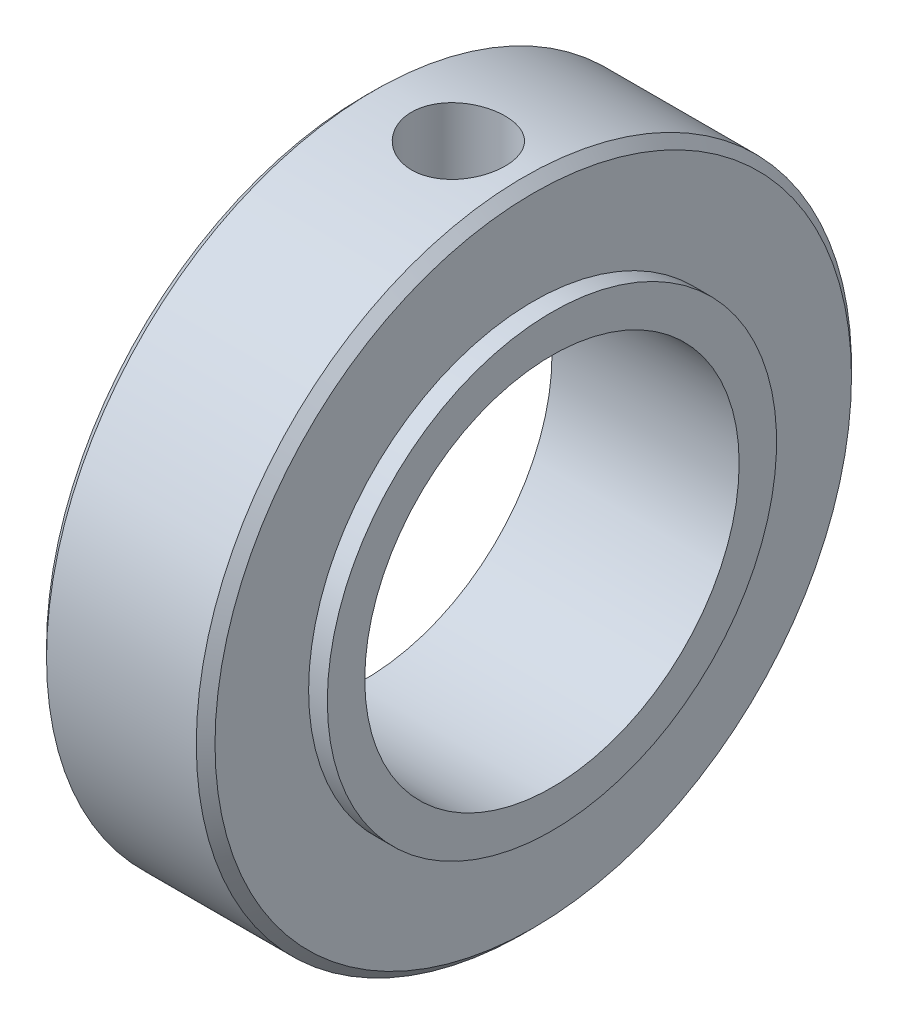
SolidWorks part; units mm, degrees
ref_plane "Front Plane" through (0, 0, 0) normal (0, 0, 1) x (1, 0, 0)
ref_plane "Top Plane" through (0, 0, 0) normal (0, 1, 0) x (1, 0, 0)
ref_plane "Right Plane" through (0, 0, 0) normal (1, 0, 0) x (0, 0, -1)
sketch "Sketch1" plane through (0, 0, 0) normal (0, 0, 1) x (1, 0, 0)
  line L0 (0, 0) -> (31.7168, 0) construction
  line L2 (0, 10) -> (10, 10)
  line L3 (0, 10) -> (0, 17.5)
  line L4 (0, 17.5) -> (9, 17.5)
  line L5 (10, 10) -> (10, 12)
  line L6 (10, 12) -> (9, 12)
  line L9 (9, 12) -> (9, 17.5)
  dimension "D1" = 20
  dimension "D2" = 24
  dimension "D3" = 35
  dimension "D4" = 1
  dimension "D5" = 10
revolve "Revolve1" add sketch "Sketch1" angle 360 about L0
hole_wizard "M6 Tapped Hole1" positions "3DSketch1" profile "Sketch2" tap size "M6" standard "GB"
sketch3d "3DSketch1"
  point P0 (5, 17.5, 0)
  point P2 (-19.3927, -13.8955, 0)
sketch "Sketch2" plane through (5, 17.5, 0) normal (1, 0, 0) x (0, 0, 1)
  line L0 (0, 0) -> (0, 16.5022)
  line L1 (0, 16.5022) -> (2.5, 15)
  line L2 (2.5, 15) -> (2.5, 0)
  line L5 (2.5, 0) -> (0, 0)
  line L10 (0, 16.5022) -> (-2.5, 15) construction
  line L11 (0, -6.35) -> (0, 107.95) construction
  dimension "螺纹孔钻头直径" = 5
  dimension "螺纹孔钻头深度" = 15
  dimension "导头角度" = 118
cosmetic thread "Cosmetic Thread2"
chamfer "Chamfer1" distance 0.5 angle 45 2 edges at (0, 0, 17.5) (9, 0, 17.5)
